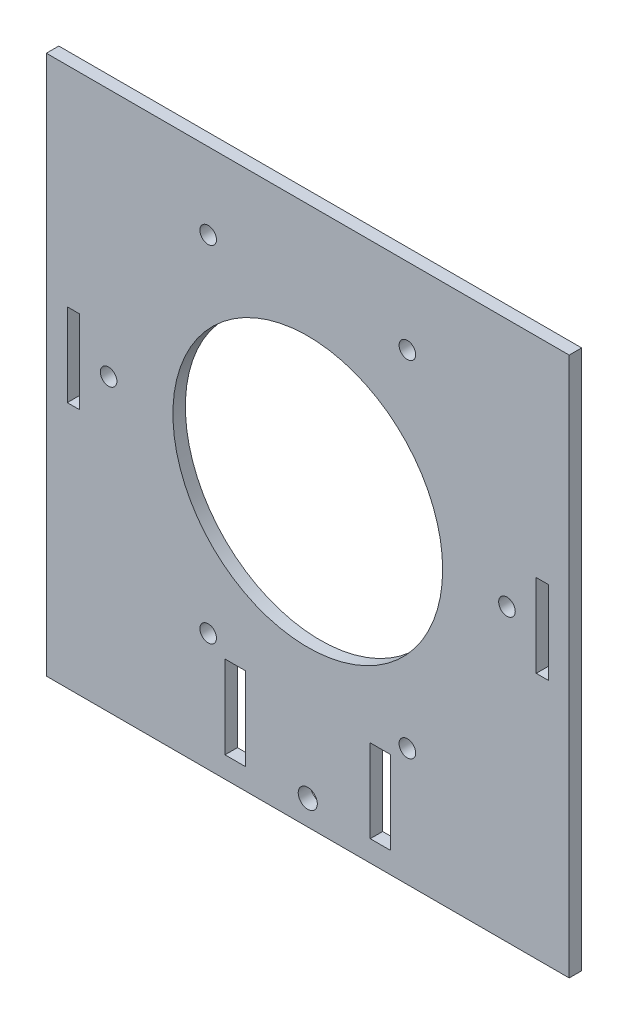
from build123d import *

# Parameters (mm, degrees)
SKETCH1_W                    = 126
SKETCH1_H                    = 130
SKETCH1_R                    = 32.5
SKETCH1_W_2                  = 4.9
SKETCH1_H_2                  = 20
BOSS_EXTRUDE1_DEPTH          = 3
SKETCH2_W                    = 2.9
SKETCH2_H                    = 20
CUT_EXTRUDE1_DEPTH           = 3
F_4_0_4_DIAMETER_HOLE1_D     = 4
F_4_0_4_DIAMETER_HOLE1_DEPTH = 10
F_4_0_4_DIAMETER_HOLE1_TIP   = 1.201721238
SKETCH6_R                    = 2.3
CUT_EXTRUDE2_DEPTH           = 3


with BuildPart() as part:
    # Sketch1 → Boss-Extrude1 (new body)
    with BuildSketch(Plane.XY):
        with Locations((0, -5)):
            Rectangle(SKETCH1_W, SKETCH1_H)
        Circle(SKETCH1_R, mode=Mode.SUBTRACT)
        with Locations((-17.5, -54.9)):
            Rectangle(SKETCH1_W_2, SKETCH1_H_2, mode=Mode.SUBTRACT)
        with Locations((17.5, -54.9)):
            Rectangle(SKETCH1_W_2, SKETCH1_H_2, mode=Mode.SUBTRACT)
    extrude(amount=BOSS_EXTRUDE1_DEPTH)

    # Sketch2 → Cut-Extrude1 (cut)
    with BuildSketch(Plane.XY.offset(3)):
        with Locations((-56.5, -0.4)):
            Rectangle(SKETCH2_W, SKETCH2_H)
    cut_extrude1 = extrude(amount=-CUT_EXTRUDE1_DEPTH, mode=Mode.SUBTRACT)

    # Mirror1: Cut-Extrude1 across plane
    add(cut_extrude1.mirror(Plane(origin=(0, 0, 0), x_dir=(0, 0, 1), z_dir=(1, 0, 0))), mode=Mode.SUBTRACT)

    # Ø4.0 (4) Diameter Hole1
    with Locations(Plane.XY.offset(3)):
        with Locations((-24, 41.569219382), (48, 0), (24, 41.569219382), (24, -41.569219382), (-24, -41.569219382), (-48, 0)):
            Hole(F_4_0_4_DIAMETER_HOLE1_D / 2, depth=F_4_0_4_DIAMETER_HOLE1_DEPTH)
            with Locations((0, 0, -(F_4_0_4_DIAMETER_HOLE1_DEPTH + F_4_0_4_DIAMETER_HOLE1_TIP / 2))):  # 118° drill point
                Cone(0, F_4_0_4_DIAMETER_HOLE1_D / 2, F_4_0_4_DIAMETER_HOLE1_TIP, mode=Mode.SUBTRACT)

    # Sketch6 → Cut-Extrude2 (cut)
    with BuildSketch(Plane.XY.offset(3)):
        with Locations((0, -64)):
            Circle(SKETCH6_R)
    extrude(amount=-CUT_EXTRUDE2_DEPTH, mode=Mode.SUBTRACT)


solid = part.part
